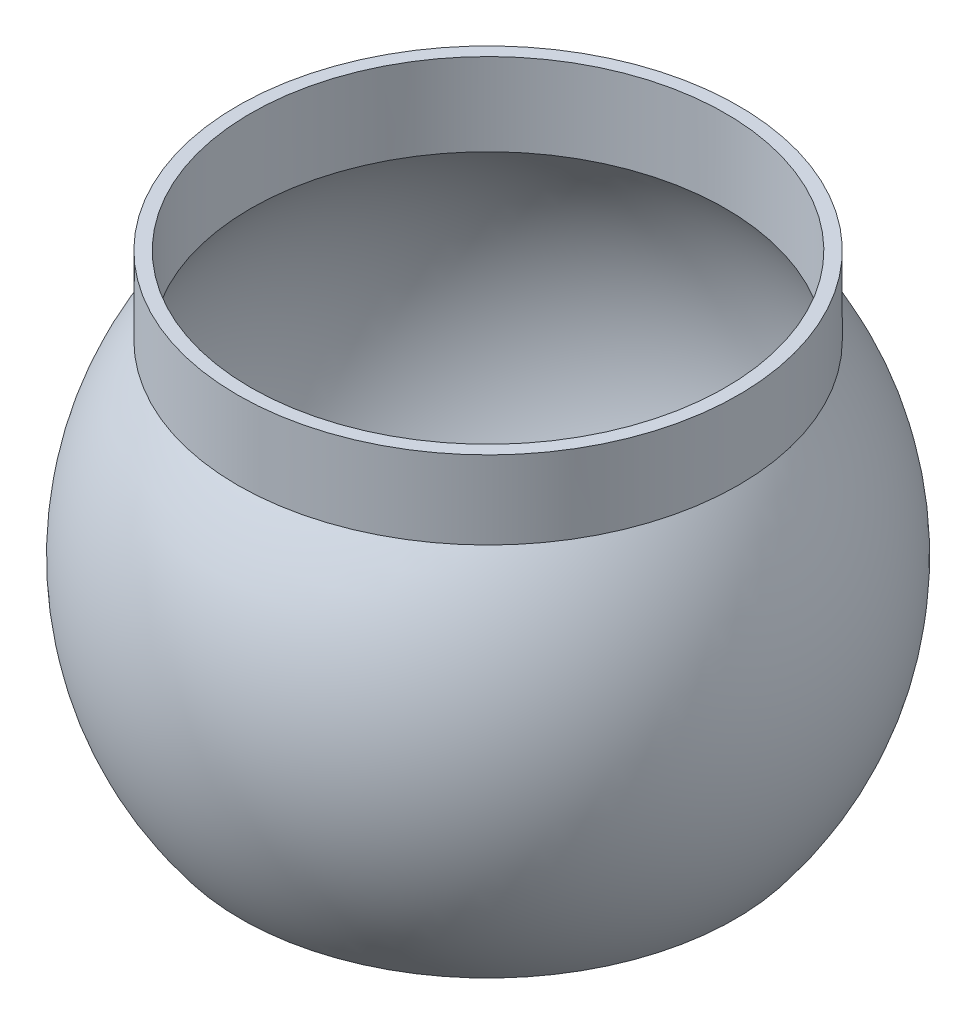
SolidWorks part; units mm, degrees
material "45"
ref_plane "前视" through (0, 0, 0) normal (0, 0, 1) x (1, 0, 0)
ref_plane "上视" through (0, 0, 0) normal (0, 1, 0) x (1, 0, 0)
ref_plane "右视" through (0, 0, 0) normal (1, 0, 0) x (0, 0, -1)
sketch "草图1" plane through (0, 0, 0) normal (0, 0, 1) x (1, 0, 0)
  line L0 (0, 0) -> (0, -67.1924) construction
  line L1 (0, 0) -> (-38.5, 0)
  line L2 (-38.5, 0) -> (-38.5, -12)
  line L3 (-37.9938, -70) -> (0, -70)
  line L4 (0, 0) -> (0, -70)
  arc A0 (-38.5, -12) -> (-37.9938, -70) centre (0, -40.6662) ccw
  dimension "D4" = 48
  dimension "D1" = 77
  dimension "D2" = 12
  dimension "D3" = 70
revolve "旋转1" add sketch "草图1" angle 360 about L0
shell "抽壳1" thickness 2
